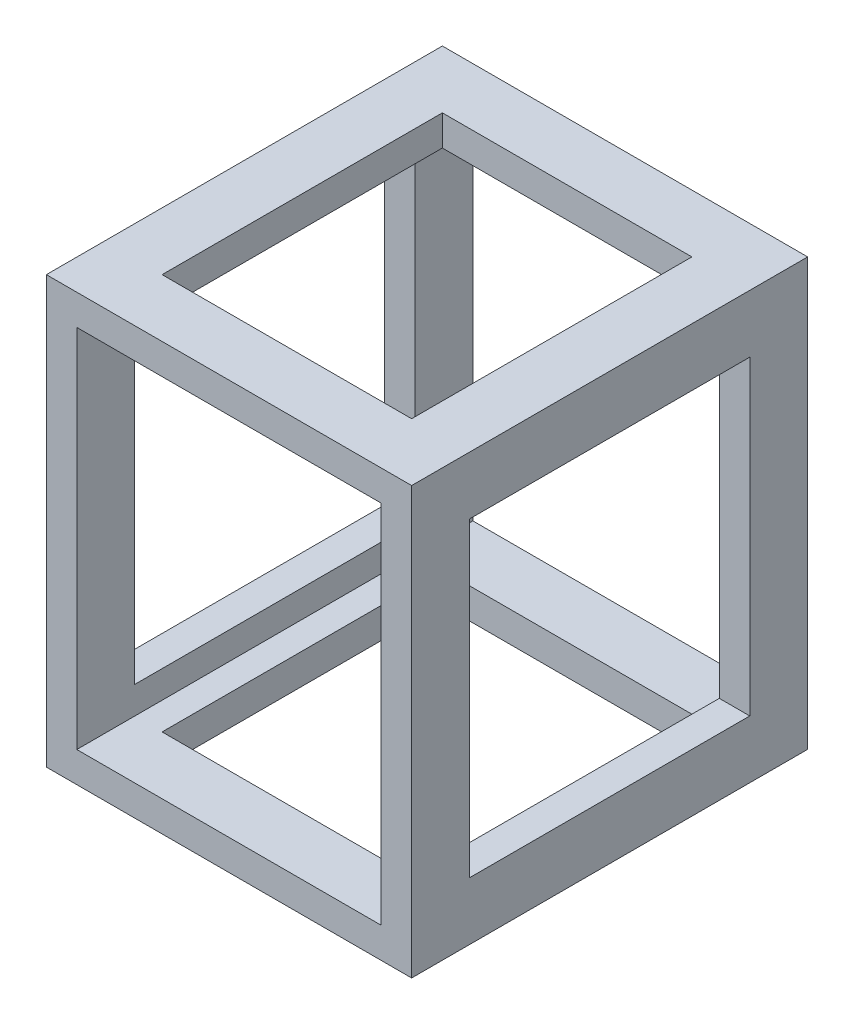
SolidWorks part; units mm, degrees
ref_plane "Front Plane" through (0, 0, 0) normal (0, 0, 1) x (1, 0, 0)
ref_plane "Top Plane" through (0, 0, 0) normal (0, 1, 0) x (1, 0, 0)
ref_plane "Right Plane" through (0, 0, 0) normal (1, 0, 0) x (0, 0, -1)
sketch "Sketch1" plane through (0, 0, 0) normal (0, 0, 1) x (1, 0, 0)
  line L0 (-70, 90) -> (49.9115, 90)
  line L1 (49.9115, 90) -> (49.9115, 230)
  line L2 (49.9115, 230) -> (-70, 230)
  line L3 (-70, 230) -> (-70, 90)
  line L4 (-60, 100) -> (39.9115, 100)
  line L5 (39.9115, 100) -> (39.9115, 220)
  line L6 (39.9115, 220) -> (-60, 220)
  line L7 (-60, 220) -> (-60, 100)
  line L8 (-60, 100) -> (39.9115, 100)
  line L9 (39.9115, 100) -> (39.9115, 220)
  line L10 (39.9115, 220) -> (-60, 220)
  line L11 (-60, 220) -> (-60, 100)
  dimension "D1" = 0
  dimension "D2" = 10
extrude "Boss-Extrude1" add sketch "Sketch1" against normal blind 130
sketch "Sketch2" plane through (0, 90, 0) normal (0, -1, 0) x (1, 0, 0)
  line L8 (30.9115, -19) -> (-51, -19)
  line L9 (-51, -19) -> (-51, -111)
  line L10 (-51, -111) -> (30.9115, -111)
  line L11 (30.9115, -111) -> (30.9115, -19)
  line L12 (30.9115, -19) -> (-51, -19)
  line L13 (-51, -19) -> (-51, -111)
  line L14 (-51, -111) -> (30.9115, -111)
  line L15 (30.9115, -111) -> (30.9115, -19)
  dimension "D1" = 19
extrude "Cut-Extrude1" cut sketch "Sketch2" against normal blind 258
sketch "Sketch3" plane through (-70, 0, 0) normal (-1, 0, 0) x (0, 0, 1)
  line L8 (-19, 109) -> (-19, 211)
  line L9 (-19, 211) -> (-111, 211)
  line L10 (-111, 211) -> (-111, 109)
  line L11 (-111, 109) -> (-19, 109)
  line L12 (-19, 109) -> (-19, 211)
  line L13 (-19, 211) -> (-111, 211)
  line L14 (-111, 211) -> (-111, 109)
  line L15 (-111, 109) -> (-19, 109)
  dimension "D1" = 19
extrude "Cut-Extrude2" cut sketch "Sketch3" against normal blind 258
